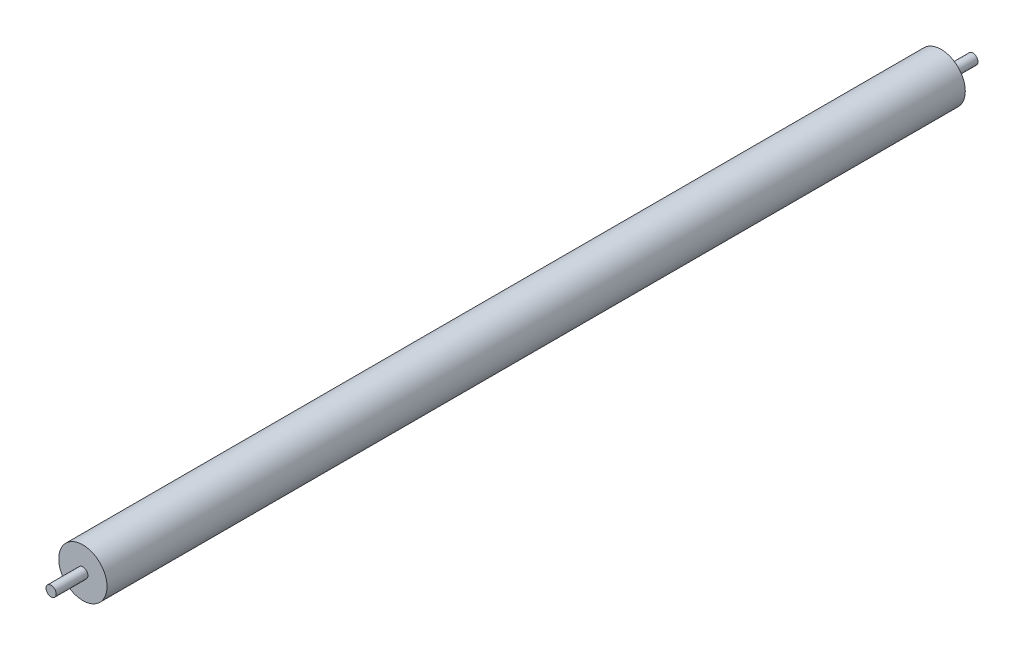
SolidWorks part; units mm, degrees
material "1060 合金"
ref_plane "前视基准面" through (0, 0, 0) normal (0, 0, 1) x (1, 0, 0)
ref_plane "上视基准面" through (0, 0, 0) normal (0, 1, 0) x (1, 0, 0)
ref_plane "右视基准面" through (0, 0, 0) normal (1, 0, 0) x (0, 0, -1)
sketch "草图1" plane through (0, 0, 0) normal (0, 0, 1) x (1, 0, 0)
  circle A0 centre (0, 0) radius 38
  dimension "D1" = 76
extrude "凸台-拉伸1" add sketch "草图1" along normal mid plane 1350
sketch "草图2" plane through (0, 0, 675) normal (0, 0, 1) x (1, 0, 0)
  circle A0 centre (0, 0) radius 8
  dimension "D1" = 16
extrude "凸台-拉伸2" add sketch "草图2" along normal mid plane 100
mirror "镜向1" about plane through (0, 0, 0) normal (0, 0, 1) of "凸台-拉伸2"
